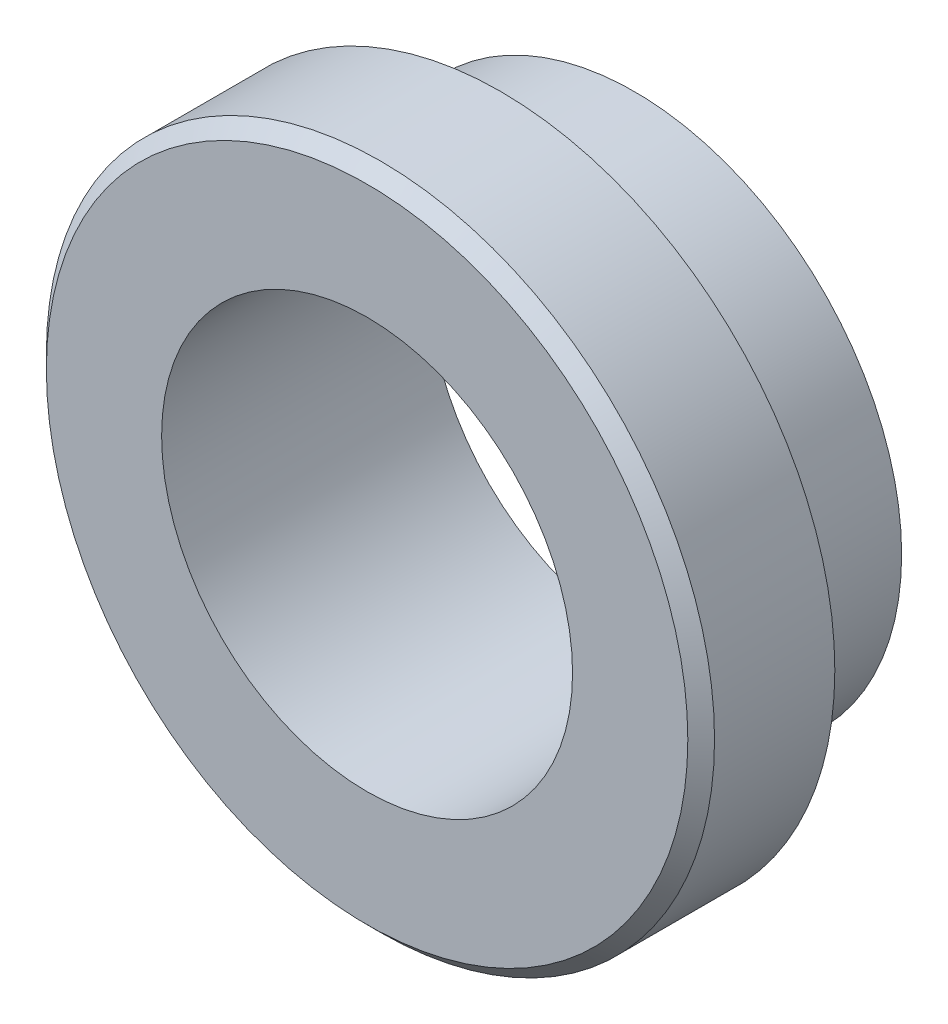
from build123d import *

# Parameters (mm, degrees)
G1_TAPPED_HOLE1_D = 30.75
CHAMFER1_SIZE     = 1


with BuildPart() as part:
    # Sketch1 → Revolve1 (revolve)
    with BuildSketch(Plane(origin=(0, 0, 0), x_dir=(0, 0, -1), z_dir=(1, 0, 0)), mode=Mode.PRIVATE) as revolve1_sk:
        Polygon((0, 0), (0, 20), (-10, 20), (-10, 25), (-20, 25), (-20, 0), align=None)
    revolve(revolve1_sk.sketch.rotate(Axis((0, 0, 20), (0, 0, -1)), 90), axis=Axis((0, 0, 20), (0, 0, -1)))

    # G1 Tapped Hole1 (through all)
    with Locations(Plane.XY.offset(20)):
        with Locations((0, 0)):
            Hole(G1_TAPPED_HOLE1_D / 2)

    # Chamfer1
    chamfer1_edges = [part.edges().sort_by_distance(p)[0] for p in [
        (-25, 0, 20),
    ]]
    chamfer(chamfer1_edges, length=CHAMFER1_SIZE)


solid = part.part
